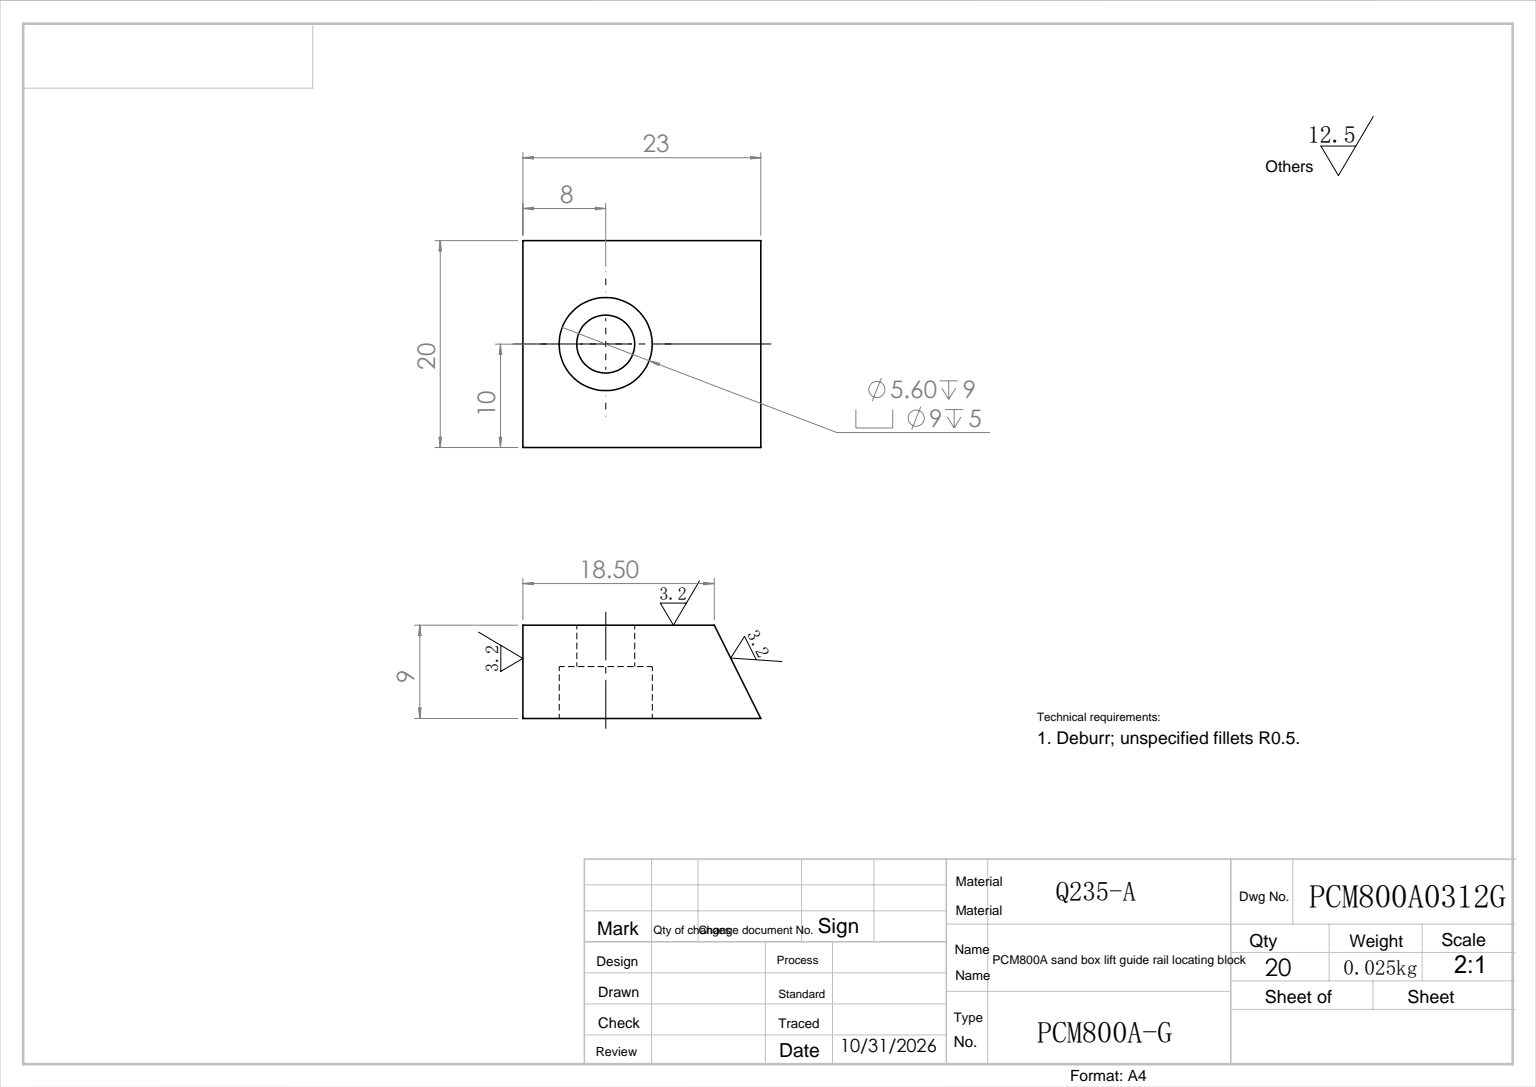
SolidWorks part; units mm, degrees
ref_plane "前视基准面" through (0, 0, 0) normal (0, 0, 1) x (1, 0, 0)
ref_plane "上视基准面" through (0, 0, 0) normal (0, 1, 0) x (1, 0, 0)
ref_plane "右视基准面" through (0, 0, 0) normal (1, 0, 0) x (0, 0, -1)
sketch "草图1" plane through (0, 0, 0) normal (0, 1, 0) x (1, 0, 0)
  line L0 (0, 0) -> (18.5, 0)
  line L1 (0, 0) -> (0, 9)
  line L2 (0, 9) -> (23, 9)
  line L3 (18.5, 0) -> (23, 9)
  dimension "D1" = 9
  dimension "D2" = 18.5
  dimension "D3" = 23
extrude "拉伸1" add sketch "草图1" along normal blind 20
sketch "草图2" plane through (0, 0, -9) normal (0, 0, -1) x (-1, 0, 0)
  line L0 (-8, 10) -> (-8, 20) construction
  line L1 (-23, 20) -> (0, 20) construction
  line L2 (-8, 10) -> (0, 10) construction
  line L3 (0, 20) -> (0, 0) construction
  circle A0 centre (-8, 10) radius 4.5
  dimension "D1" = 8
  dimension "D2" = 10
extrude "切除-拉伸1" cut sketch "草图2" against normal blind 5
sketch "草图3" plane through (0, 0, -4) normal (0, 0, -1) x (-1, 0, 0)
  circle A0 centre (-8, 10) radius 2.8
extrude "切除-拉伸2" cut sketch "草图3" against normal through all
